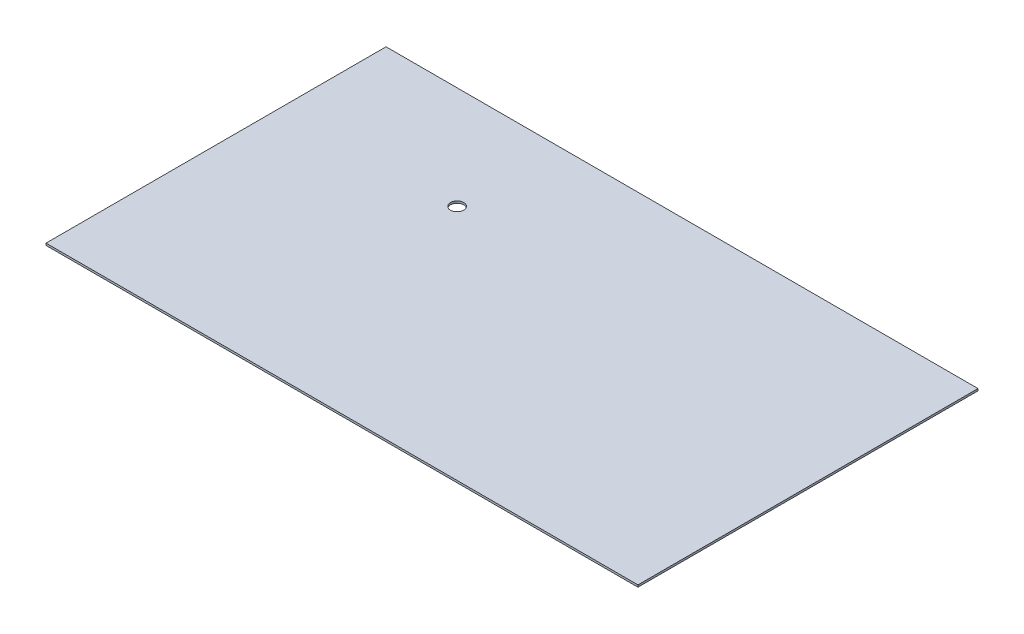
from build123d import *

# Parameters (mm, degrees)
SKETCH_1_W      = 2324
SKETCH_1_H      = 1335
SKETCH_1_R      = 26
EXTRUDE_1_DEPTH = 4


with BuildPart() as part:
    # 草图1 → 凸台-拉伸1 (new, symmetric)
    with BuildSketch(Plane(origin=(0, 0, 0), x_dir=(1, 0, 0), z_dir=(0, 1, 0))):
        Rectangle(SKETCH_1_W, SKETCH_1_H)
        with Locations(Location((-480, 264.5, 0), (0, 0, 270))):
            Circle(SKETCH_1_R, mode=Mode.SUBTRACT)
    extrude(amount=EXTRUDE_1_DEPTH, both=True)


solid = part.part
